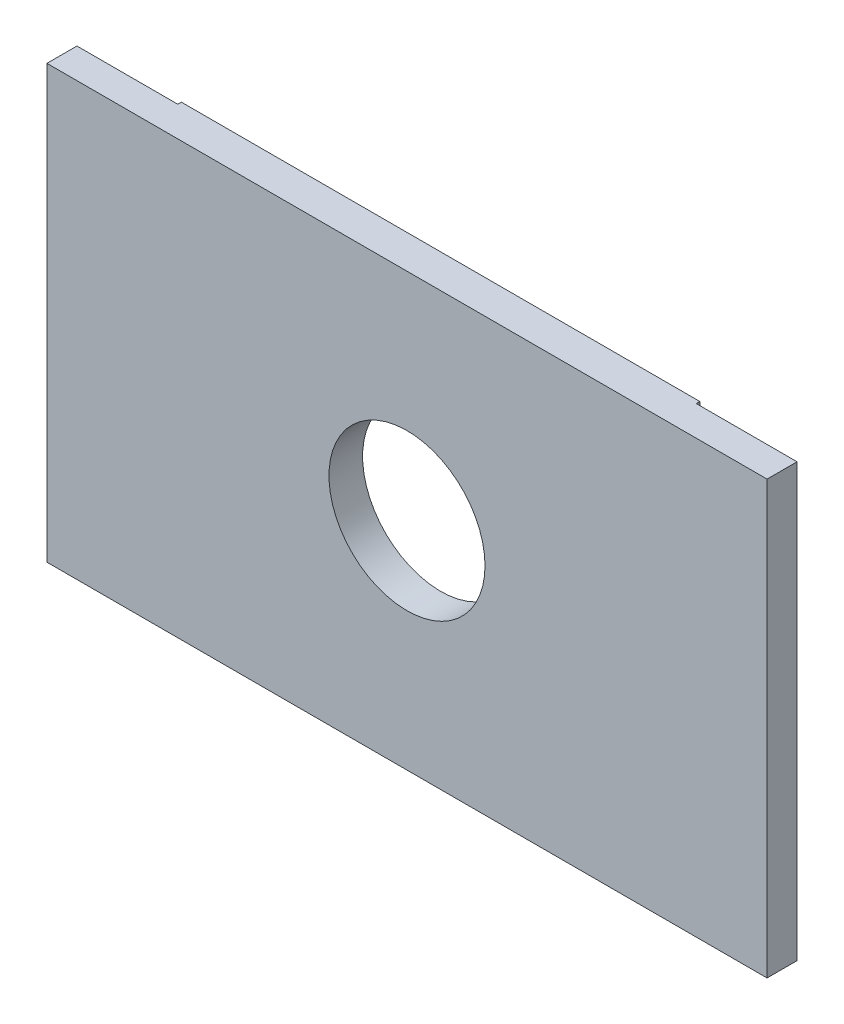
SolidWorks part; units mm, degrees
ref_plane "前视基准面" through (0, 0, 0) normal (0, 0, 1) x (1, 0, 0)
ref_plane "上视基准面" through (0, 0, 0) normal (0, 1, 0) x (1, 0, 0)
ref_plane "右视基准面" through (0, 0, 0) normal (1, 0, 0) x (0, 0, -1)
sketch "草图1" plane through (0, 0, 0) normal (0, 0, 1) x (1, 0, 0)
  line L1 (-150, -90) -> (150, -90)
  line L2 (-150, -90) -> (-150, 90)
  line L3 (-150, 90) -> (150, 90)
  line L4 (150, -90) -> (150, 90)
  line L5 (-150, -90) -> (150, 90) construction
  line L6 (-150, 90) -> (150, -90) construction
  point P0 (0, 0)
  dimension "D1" = 300
  dimension "D2" = 180
extrude "凸台-拉伸1" add sketch "草图1" along normal blind 14
sketch "草图2" plane through (0, 0, 0) normal (0, 0, -1) x (-1, 0, 0)
  line L0 (-150, 90) -> (150, 90) construction
  line L1 (150, -90) -> (108, -90)
  line L2 (150, -90) -> (150, 90)
  line L3 (150, 90) -> (108, 90)
  line L4 (108, -90) -> (108, 90)
  line L6 (-150, -90) -> (-108, -90)
  line L7 (-150, -90) -> (-150, 90)
  line L8 (-150, 90) -> (-108, 90)
  line L9 (-108, -90) -> (-108, 90)
  dimension "D1" = 42
extrude "切除-拉伸1" cut sketch "草图2" against normal blind 1.5
sketch "草图3" plane through (0, 0, 14) normal (0, 0, 1) x (1, 0, 0)
  circle A0 centre (0, 0) radius 32.5
  dimension "D1" = 65
extrude "切除-拉伸2" cut sketch "草图3" against normal up to next
